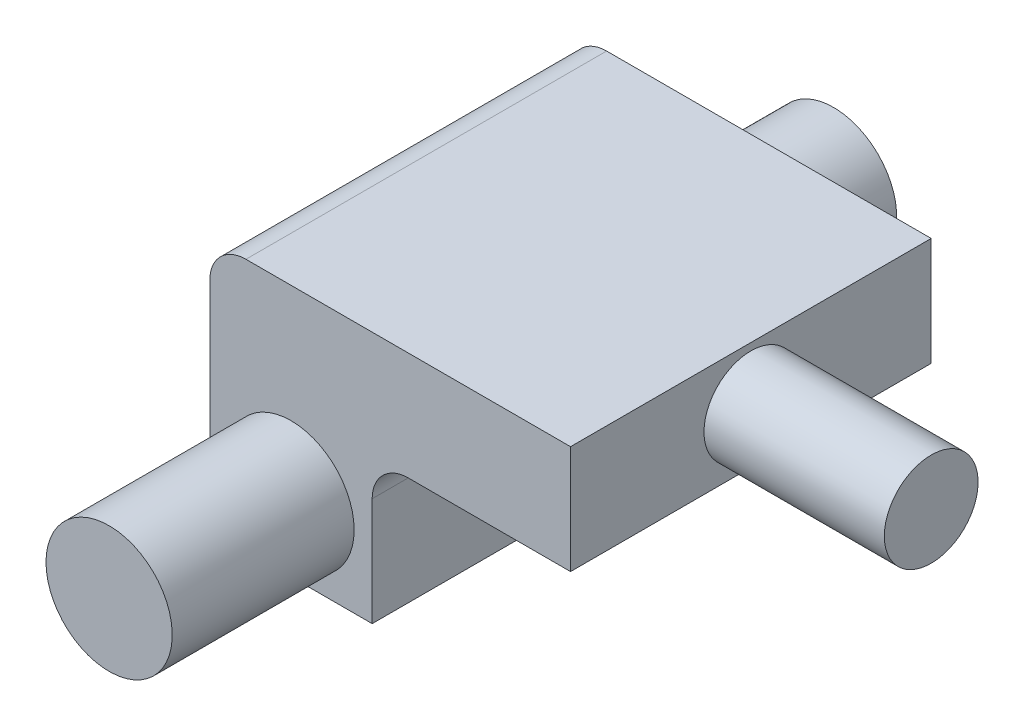
from build123d import *

# Parameters (mm, degrees)
SKETCH1_W           = 100
SKETCH1_H           = 100
BOSS_EXTRUDE1_DEPTH = 70
SKETCH2_W           = 55
SKETCH2_H           = 40
CUT_EXTRUDE1_DEPTH  = 137.037678604
SKETCH3_W           = 50
SKETCH3_H           = 13
SKETCH4_W           = 17.5
SKETCH4_H           = 50.435
SKETCH5_W           = 17.5
SKETCH5_H           = 50.435
FILLET1_R           = 10


with BuildPart() as part:
    # Sketch1 → Boss-Extrude1 (new body)
    with BuildSketch(Plane.XZ.offset(20)):
        with Locations((27.5, 0)):
            Rectangle(SKETCH1_W, SKETCH1_H)
    extrude(amount=-BOSS_EXTRUDE1_DEPTH)

    # Sketch2 → Cut-Extrude1 (cut, through all)
    with BuildSketch(Plane(origin=(0, 0, -50), x_dir=(-1, 0, 0), z_dir=(0, 0, -1))):
        with Locations((-50, 0)):
            Rectangle(SKETCH2_W, SKETCH2_H)
    extrude(amount=-CUT_EXTRUDE1_DEPTH, mode=Mode.SUBTRACT)

    # Sketch3 → Revolve1 (revolve)
    with BuildSketch(Plane(origin=(0, 0, 0), x_dir=(-1, 0, 0), z_dir=(0, 0, -1)), mode=Mode.PRIVATE) as revolve1_sk:
        with Locations((-102.5, 41.5)):
            Rectangle(SKETCH3_W, SKETCH3_H)
    revolve(revolve1_sk.sketch.rotate(Axis((127.5, 35, 0), (-1, 0, 0)), 270), axis=Axis((127.5, 35, 0), (-1, 0, 0)))

    # Sketch4 → Revolve2 (revolve)
    with BuildSketch(Plane.XZ, mode=Mode.PRIVATE) as revolve2_sk:
        with Locations((8.75, -75.2175)):
            Rectangle(SKETCH4_W, SKETCH4_H)
    revolve(revolve2_sk.sketch.rotate(Axis((0, 0, -50), (0, 0, -1)), 180), axis=Axis((0, 0, -50), (0, 0, -1)))

    # Sketch5 → Revolve3 (revolve)
    with BuildSketch(Plane.XZ, mode=Mode.PRIVATE) as revolve3_sk:
        with Locations((8.75, 75.2175)):
            Rectangle(SKETCH5_W, SKETCH5_H)
    revolve(revolve3_sk.sketch.rotate(Axis((0, 0, 100.435), (0, 0, -1)), 180), axis=Axis((0, 0, 100.435), (0, 0, -1)))

    # Fillet1
    fillet1_edges = [part.edges().sort_by_distance(p)[0] for p in [
        (22.5, 20, 0),
        (-22.5, 50, 0),
    ]]
    fillet(fillet1_edges, radius=FILLET1_R)


solid = part.part
